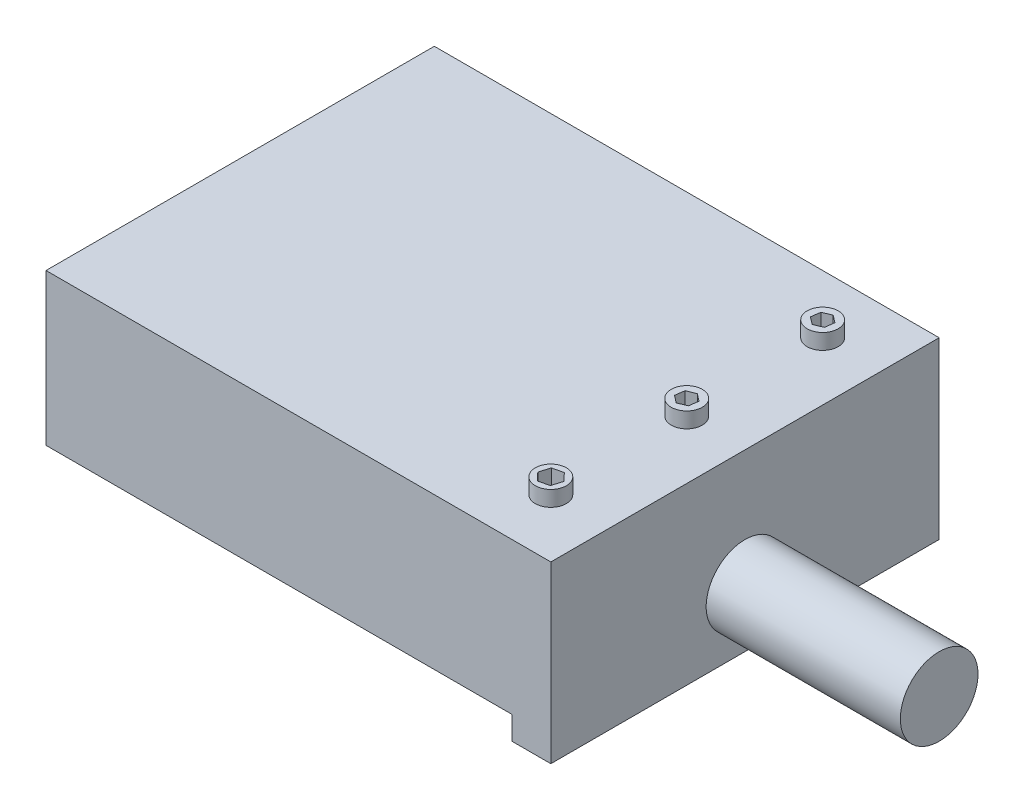
SolidWorks part; units mm, degrees
ref_plane "Front Plane" through (0, 0, 0) normal (0, 0, 1) x (1, 0, 0)
ref_plane "Top Plane" through (0, 0, 0) normal (0, 1, 0) x (1, 0, 0)
ref_plane "Right Plane" through (0, 0, 0) normal (1, 0, 0) x (0, 0, -1)
other "Configuration Table"
sketch "Sketch1" plane through (0, 0, 0) normal (0, 1, 0) x (1, 0, 0)
  line L1 (-35, 50) -> (35, 50)
  line L2 (-35, 50) -> (-35, -50)
  line L3 (-35, -50) -> (35, -50)
  line L4 (35, 50) -> (35, -50)
  line L5 (-35, 50) -> (35, -50) construction
  line L6 (-35, -50) -> (35, 50) construction
  point P0 (0, 0)
  dimension "D1" = 70
  dimension "D2" = 100
extrude "Boss-Extrude1" add sketch "Sketch1" along normal blind 30
sketch "Sketch2" plane through (0, 30, 0) normal (0, 1, 0) x (1, 0, 0)
  line L0 (20, 50) -> (20, -35) construction
  line L1 (35, 50) -> (-35, 50) construction
  line L2 (20, -35) -> (-35, -35) construction
  line L3 (-35, 50) -> (-35, -50) construction
  line L4 (35, -50) -> (35, 50) construction
  line L5 (-35, -50) -> (35, -50) construction
  line L7 (21.9131, 33.5347) -> (22.2255, 35.9241)
  line L8 (22.2255, 35.9241) -> (20.3125, 37.3894)
  line L9 (20.3125, 37.3894) -> (18.0869, 36.4653)
  line L10 (18.0869, 36.4653) -> (17.7745, 34.0759)
  line L11 (17.7745, 34.0759) -> (19.6875, 32.6106)
  line L12 (19.6875, 32.6106) -> (21.9131, 33.5347)
  line L13 (21.9131, -1.4702) -> (22.2298, 0.9217)
  line L14 (22.2298, 0.9217) -> (20.3167, 2.3919)
  line L15 (20.3167, 2.3919) -> (18.0869, 1.4702)
  line L16 (18.0869, 1.4702) -> (17.7702, -0.9217)
  line L17 (17.7702, -0.9217) -> (19.6833, -2.3919)
  line L18 (19.6833, -2.3919) -> (21.9131, -1.4702)
  line L19 (21.9131, -37.0352) -> (22.719, -34.3608)
  line L20 (22.719, -34.3608) -> (20.806, -32.3257)
  line L21 (20.806, -32.3257) -> (18.0869, -32.9648)
  line L22 (18.0869, -32.9648) -> (17.281, -35.6392)
  line L23 (17.281, -35.6392) -> (19.194, -37.6743)
  line L24 (19.194, -37.6743) -> (21.9131, -37.0352)
  circle A1 centre (20, -35) radius 4
  circle A2 centre (20, 0) radius 4
  circle A3 centre (20, 35) radius 4
  circle A4 centre (20, 35) radius 2.0869 construction
  circle A5 centre (20, 0) radius 2.0895 construction
  circle A6 centre (20, -35) radius 2.4189 construction
  dimension "D4" = 8
  dimension "D5" = 8
  dimension "D6" = 8
  dimension "D1" = 15
  dimension "D2" = 15
  dimension "D8" = 35
  dimension "D9" = 35
extrude "Boss-Extrude2" add sketch "Sketch2" along normal blind 4
sketch "Sketch3" plane through (35, 0, 0) normal (1, 0, 0) x (0, 0, -1)
  line L0 (-50, 30) -> (50, 30) construction
  circle A0 centre (0, 0) radius 10
  dimension "D1" = 20
  dimension "D2" = 30
extrude "Boss-Extrude3" add sketch "Sketch3" along normal blind 50
sketch "Sketch4" plane through (0, 0, 0) normal (0, -1, 0) x (1, 0, 0)
  line L1 (-35, 50) -> (35, 50)
  line L2 (-35, 50) -> (-35, -50)
  line L3 (-35, -50) -> (35, -50)
  line L4 (35, 50) -> (35, -50)
extrude "Boss-Extrude4" add sketch "Sketch4" along normal blind 15
sketch "Sketch5" plane through (0, 0, -50) normal (0, 0, -1) x (-1, 0, 0)
  line L1 (35, -15) -> (-25, -15)
  line L2 (35, -15) -> (35, -9)
  line L3 (35, -9) -> (-25, -9)
  line L4 (-25, -15) -> (-25, -9)
  dimension "D1" = 60
  dimension "D2" = 6
extrude "Cut-Extrude1" cut sketch "Sketch5" against normal up to next
sketch "Sketch6" plane through (-35, 0, 0) normal (-1, 0, 0) x (0, 0, 1)
  line L1 (-50, -9) -> (50, -9)
  line L2 (-50, -9) -> (-50, 30)
  line L3 (-50, 30) -> (50, 30)
  line L4 (50, -9) -> (50, 30)
extrude "Boss-Extrude5" add sketch "Sketch6" along normal blind 60
